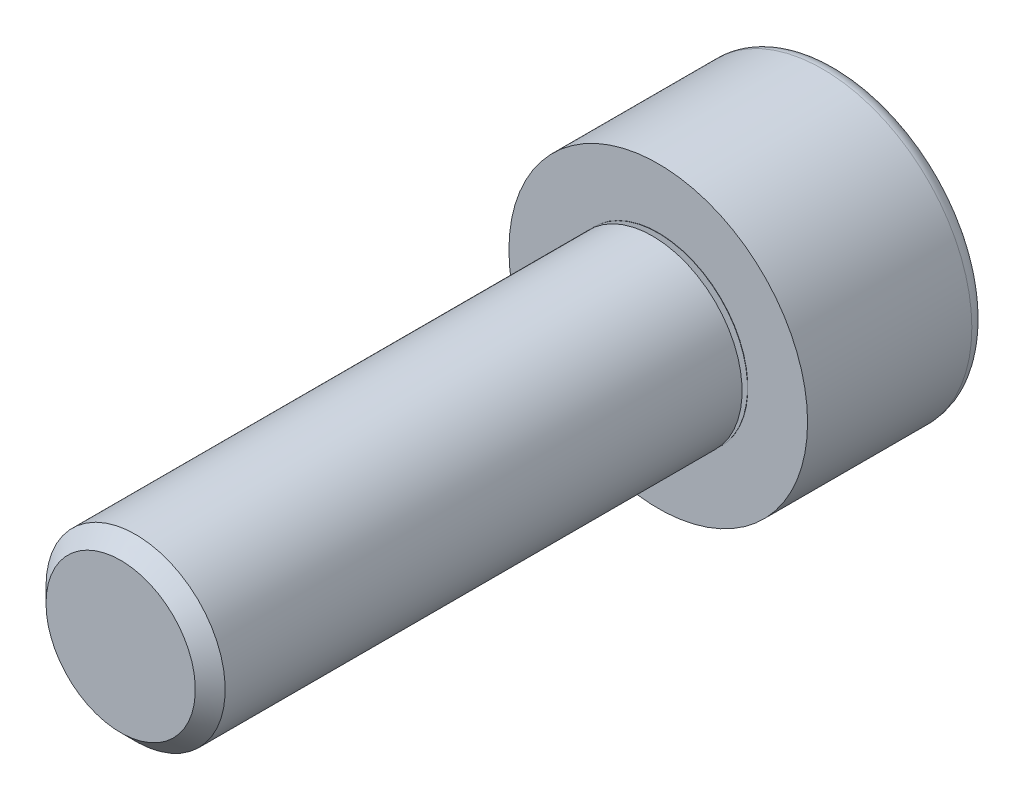
SolidWorks part; units mm, degrees
ref_plane "Front" through (0, 0, 0) normal (0, 0, 1) x (1, 0, 0)
ref_plane "Top" through (0, 0, 0) normal (0, 1, 0) x (1, 0, 0)
ref_plane "Right" through (0, 0, 0) normal (1, 0, 0) x (0, 0, -1)
sketch "Logo3_Revol_Axis" plane through (0, 0, 0) normal (0, 1, 0) x (1, 0, 0)
  line L0 (0, -43.5172) -> (0, 43.5172) construction
sketch "Logo3_bib1" plane through (0, 0, 0) normal (0, -1, 0) x (-1, 0, 0)
  line L0 (0, -18) -> (0, 6)
  line L1 (0, 6) -> (4.5, 6)
  line L2 (5, 5.5) -> (5, 0)
  line L3 (5, 0) -> (3, 0)
  line L4 (3, 0) -> (3, -0.01)
  line L5 (3, -17.5) -> (2.5, -18)
  line L6 (2.5, -18) -> (0, -18)
  line L7 (3, -0.01) -> (2.6134, -0.01)
  line L8 (2.6066, -0.0488) -> (3, -0.192)
  line L9 (3, -0.192) -> (3, -17.5)
  line L10 (0, 10.5852) -> (0, -63.2873) construction
  arc A0 (4.5, 6) -> (5, 5.5) centre (4.5, 5.5) cw
  arc A1 (2.6134, -0.01) -> (2.6066, -0.0488) centre (2.6134, -0.03) ccw
  point P17 (2.5, -0.01)
revolve "Revolve1" add sketch "Logo3_bib1" angle 360 about L10
cosmetic thread "Cosmetic Thread1"
sketch "Logo3_bib2" plane through (0, 0, -6) normal (0, 0, -1) x (1, 0, 0)
  line L1 (2.8868, 0) -> (1.4434, 2.5)
  line L2 (1.4434, 2.5) -> (-1.4434, 2.5)
  line L3 (-1.4434, 2.5) -> (-2.8868, 0)
  line L4 (-2.8868, 0) -> (-1.4434, -2.5)
  line L5 (-1.4434, -2.5) -> (1.4434, -2.5)
  line L6 (1.4434, -2.5) -> (2.8868, 0)
  circle A0 centre (0, 0) radius 2.5 construction
extrude "Cut-Extrude1" cut sketch "Logo3_bib2" against normal blind 2.5
equation "\"DIA2@XZQB7_bib1\" = \"XZQB7_d1-pas@XZQB7_bib1\""
equation "\"LGT1@XZQB7_bib1\" = \"XZQB7_d1@XZQB7_bib1\""
equation "\"D1@Cut-Extrude1\" = \"XZQB7_c1@XZQB7_bib2\"/2."
equation "\"D2@Cosmetic Thread1\" = \"XZQB7_d1-pas@XZQB7_bib1\""
